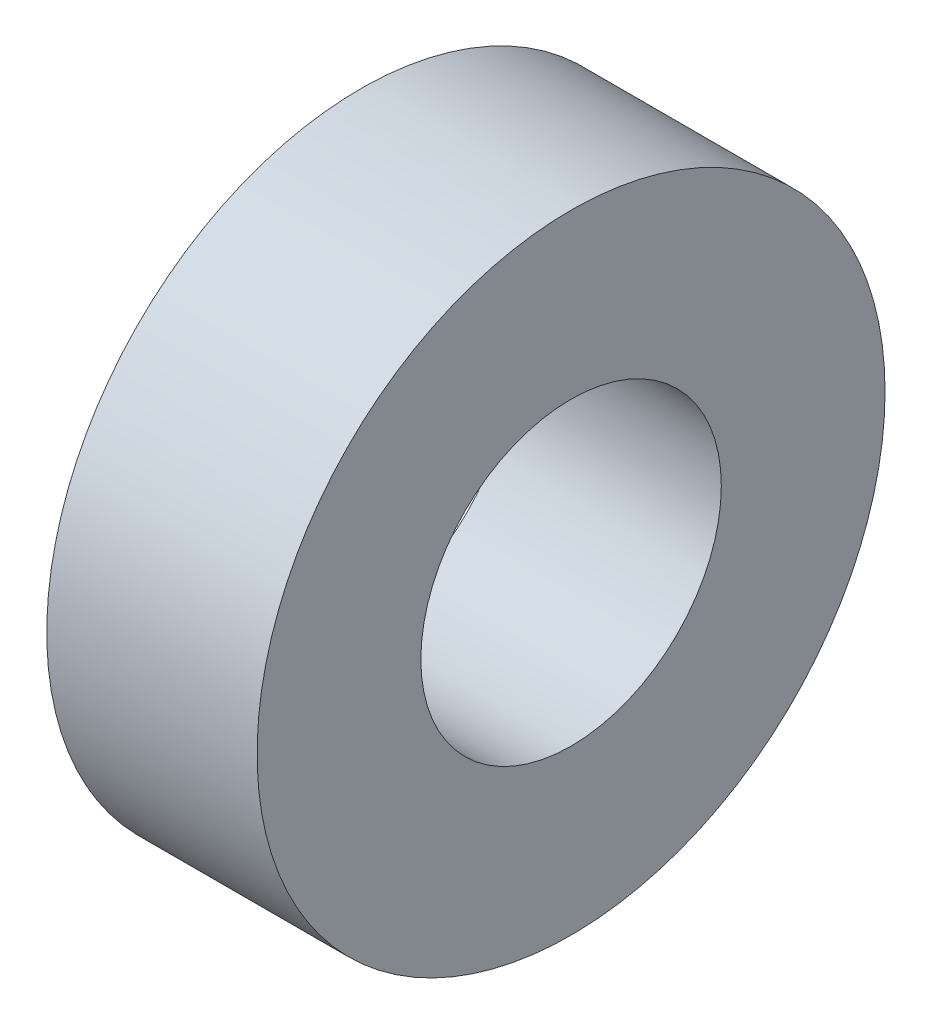
SolidWorks part; units mm, degrees
material "6061-T6 (SS)"
ref_plane "前视基准面" through (0, 0, 0) normal (0, 0, 1) x (1, 0, 0)
ref_plane "上视基准面" through (0, 0, 0) normal (0, 1, 0) x (1, 0, 0)
ref_plane "右视基准面" through (0, 0, 0) normal (1, 0, 0) x (0, 0, -1)
other "Configuration Table"
sketch "草图1" plane through (0, 0, 0) normal (1, 0, 0) x (0, 0, -1)
  circle A0 centre (0, 0) radius 41.8
  circle A1 centre (0, 0) radius 20
  dimension "D1" = 83.6
  dimension "D2" = 40
extrude "凸台-拉伸1" add sketch "草图1" along normal blind 28
